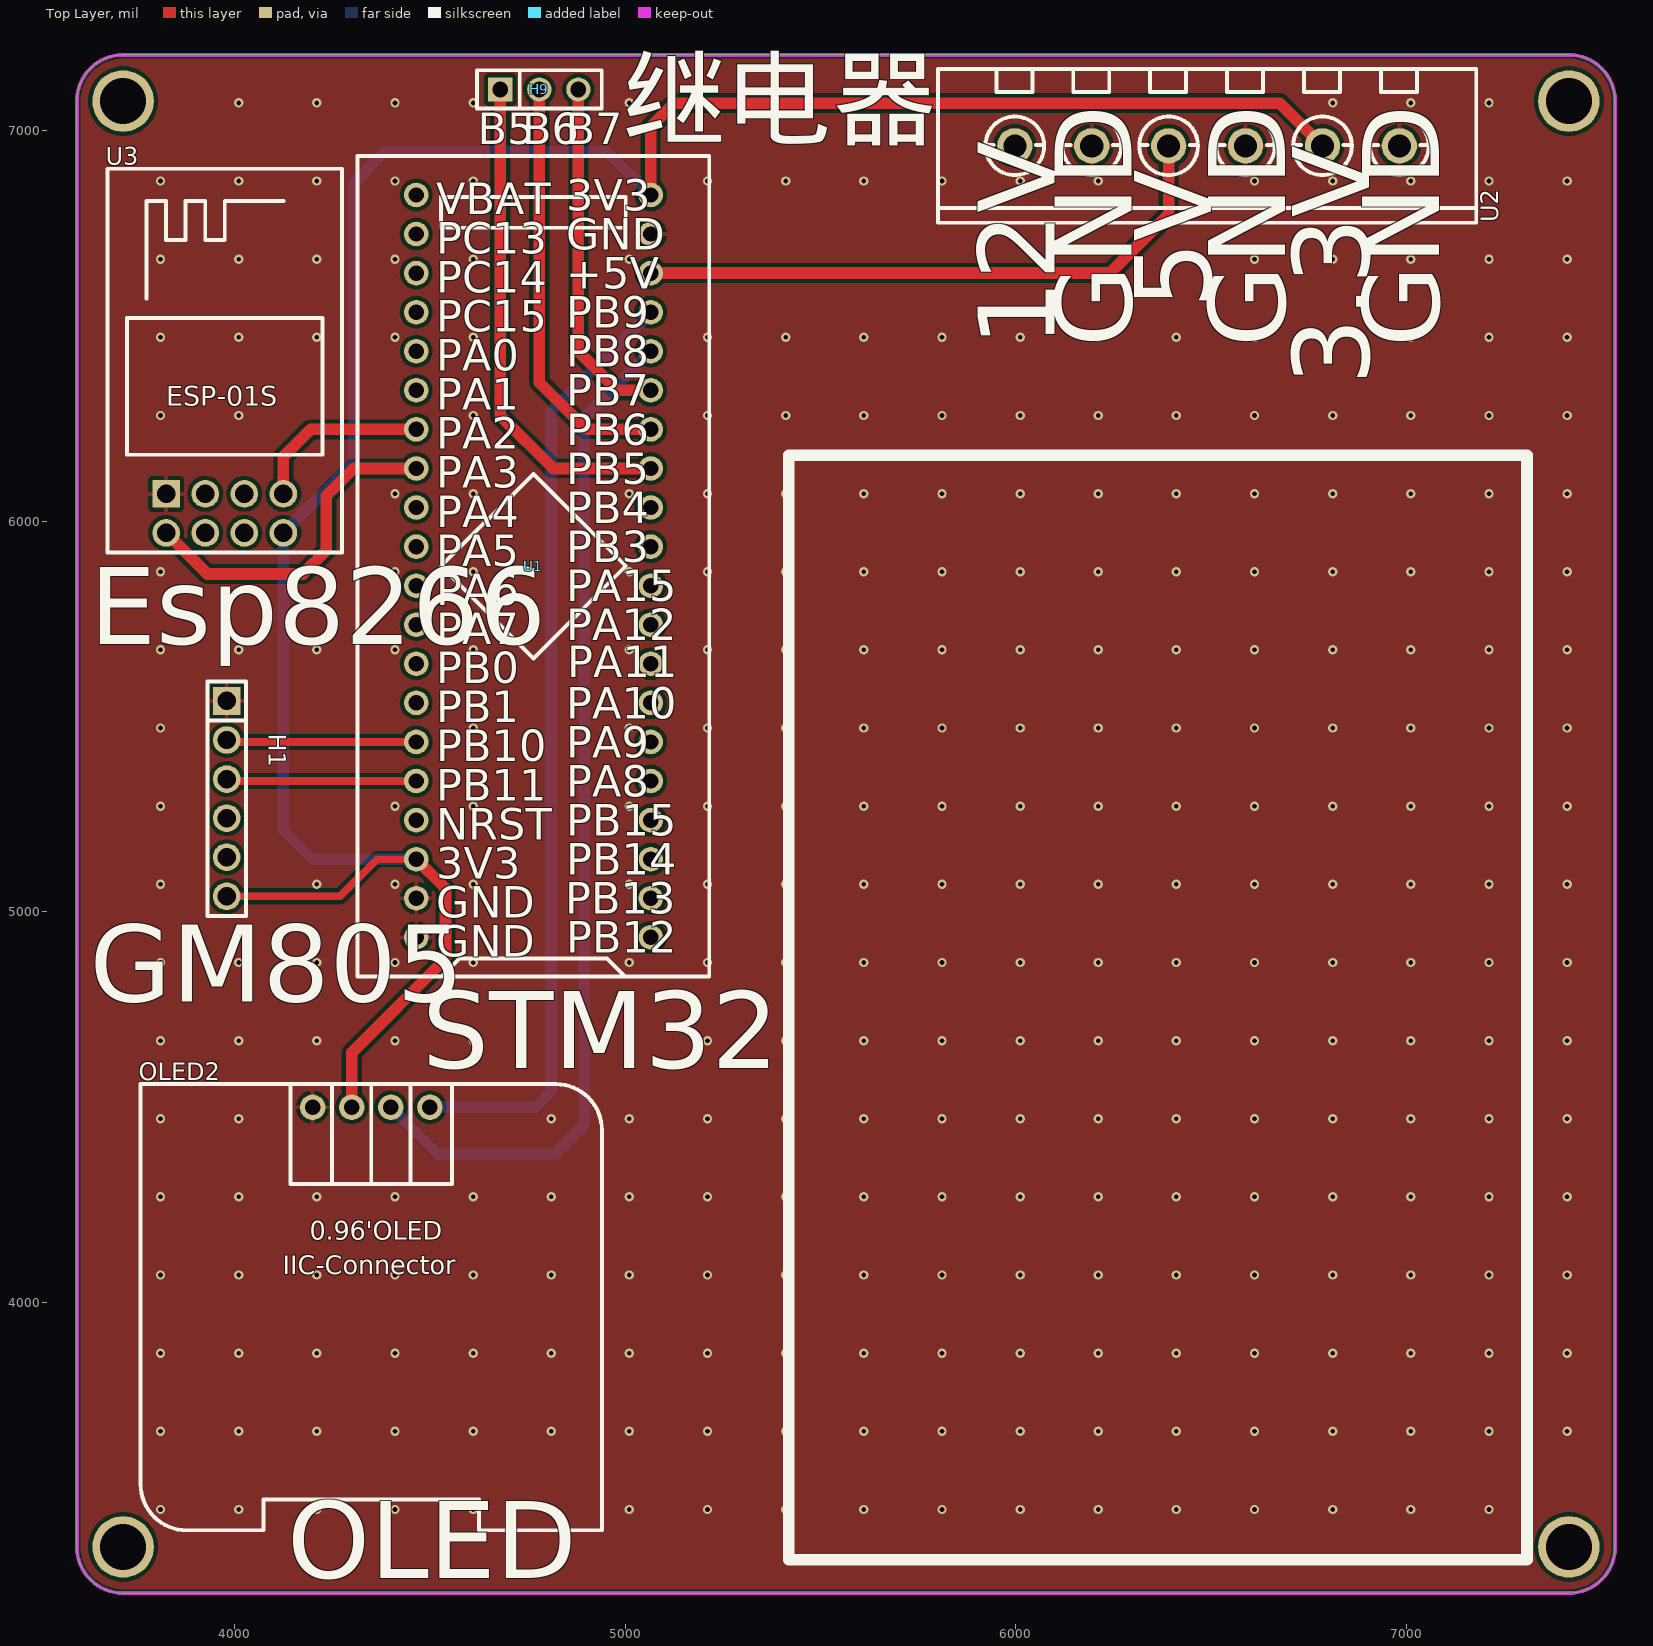
[diagram p0: Top Layer view]
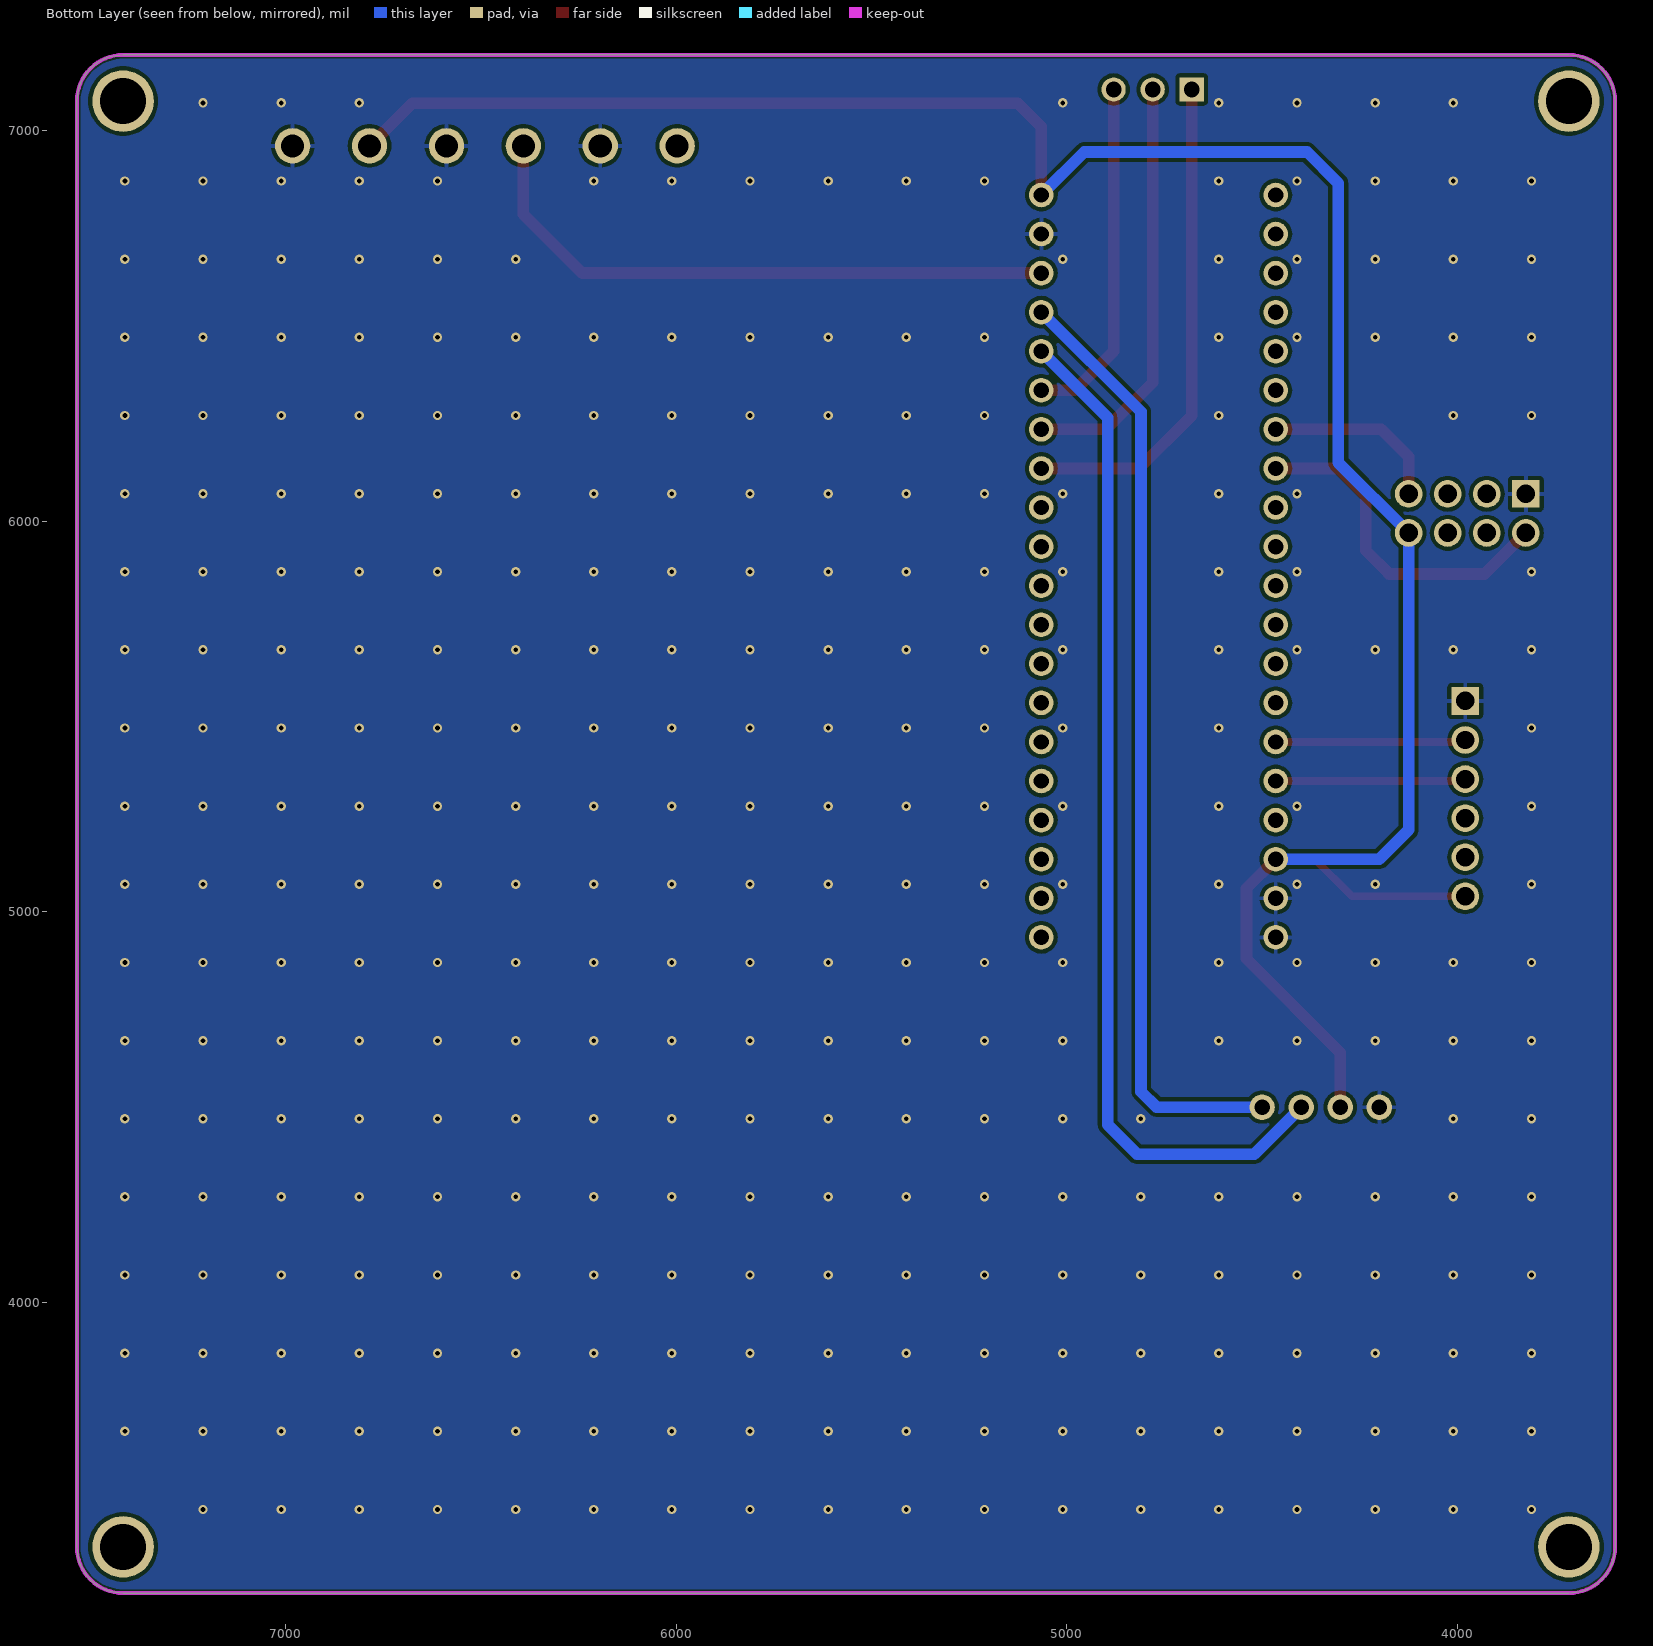
[diagram p1: Bottom Layer view, seen from below]
# Altium PCB MISC52106.pcbdoc
Units mil, origin at the board's own origin, x right, y up, seen from the top; angles counter-clockwise.
Board outline 3937.01 x 3937.01 mil, 2 copper layers (Top Layer, Bottom Layer), stack 62.206 mil thick; 6 components, 38 nets, 71 pads, 311 vias.

## Layer stack, top to bottom
Top Solder Mask Layer: solder mask 0.394, Dk 3.3
Top Layer: signal copper 1.379
Dielectric1: surface 59.449, FR4, Dk 4.5
Bottom Layer: signal copper 1.378
Bottom Solder Mask Layer: solder mask 0.394, Dk 3.3

## Board outline
3714.61,7193.5 ccw(c3714.61,7075.39) 3596.5,7075.39 3596.5,3374.61 ccw(c3714.61,3374.61) 3714.61,3256.5 7415.39,3256.5 ccw(c7415.39,3374.61) 7533.5,3374.61 7533.5,7075.39 ccw(c7415.39,7075.39) 7415.39,7193.5 3714.61,7193.5

## Design rules (kind name [scope] priority, off if disabled: settings)
BoardOutlineClearance copperThickness2oz_1 [All] p2 off: genericclearance=7.99 ignorepadtopadclearanceinfootprint=FALSE except(0: Arc-SplitContinuation Track-SplitContinuation SMDPad-SplitContinuation THPad-SplitContinuation Via-SplitContinuation Fill-SplitContinuation Region-SplitContinuation Poly-SplitContinuation Text-SplitContinuation Hole-SplitContinuation; 5.98: Arc-CutoutEdge Track-CutoutEdge SMDPad-CutoutEdge THPad-CutoutEdge Via-CutoutEdge Text-CutoutEdge; 6.9: Hole-OutlineEdge Hole-CutoutEdge; 10: Poly-OutlineEdge Poly-CutoutEdge; 11.81: Arc-OutlineEdge Track-OutlineEdge SMDPad-OutlineEdge THPad-OutlineEdge Via-OutlineEdge Fill-OutlineEdge Region-OutlineEdge Text-OutlineEdge Fill-CutoutEdge Region-CutoutEdge)
BoardOutlineClearance Plane_innerPlane_1 [All] p4 off: genericclearance=4.02 ignorepadtopadclearanceinfootprint=FALSE except(0: Arc-SplitContinuation Track-SplitContinuation SMDPad-SplitContinuation THPad-SplitContinuation Via-SplitContinuation Fill-SplitContinuation Region-SplitContinuation Poly-SplitContinuation Text-SplitContinuation Hole-SplitContinuation; 5.98: Arc-CutoutEdge Track-CutoutEdge SMDPad-CutoutEdge THPad-CutoutEdge Via-CutoutEdge Text-CutoutEdge; 6.9: Hole-OutlineEdge Hole-CutoutEdge; 10: Poly-OutlineEdge Poly-CutoutEdge; 11.81: Arc-OutlineEdge Track-OutlineEdge SMDPad-OutlineEdge THPad-OutlineEdge Via-OutlineEdge Fill-OutlineEdge Region-OutlineEdge Text-OutlineEdge Fill-CutoutEdge Region-CutoutEdge)
BoardOutlineClearance Copper_copperRegion_1 [All] p6 off: genericclearance=4.02 ignorepadtopadclearanceinfootprint=FALSE except(0: Arc-SplitContinuation Track-SplitContinuation SMDPad-SplitContinuation THPad-SplitContinuation Via-SplitContinuation Fill-SplitContinuation Region-SplitContinuation Poly-SplitContinuation Text-SplitContinuation Hole-SplitContinuation; 5.98: Arc-CutoutEdge Track-CutoutEdge SMDPad-CutoutEdge THPad-CutoutEdge Via-CutoutEdge Text-CutoutEdge; 6.9: Hole-OutlineEdge Hole-CutoutEdge; 10: Poly-OutlineEdge Poly-CutoutEdge; 11.81: Arc-OutlineEdge Track-OutlineEdge SMDPad-OutlineEdge THPad-OutlineEdge Via-OutlineEdge Fill-OutlineEdge Region-OutlineEdge Text-OutlineEdge Fill-CutoutEdge Region-CutoutEdge)
BoardOutlineClearance Copper_copperRegion_copperThickness1oz_1 [All] p8 off: genericclearance=4.02 ignorepadtopadclearanceinfootprint=FALSE except(0: Arc-SplitContinuation Track-SplitContinuation SMDPad-SplitContinuation THPad-SplitContinuation Via-SplitContinuation Fill-SplitContinuation Region-SplitContinuation Poly-SplitContinuation Text-SplitContinuation Hole-SplitContinuation; 5.98: Arc-CutoutEdge Track-CutoutEdge SMDPad-CutoutEdge THPad-CutoutEdge Via-CutoutEdge Text-CutoutEdge; 6.9: Hole-OutlineEdge Hole-CutoutEdge; 10: Poly-OutlineEdge Poly-CutoutEdge; 11.81: Arc-OutlineEdge Track-OutlineEdge SMDPad-OutlineEdge THPad-OutlineEdge Via-OutlineEdge Fill-OutlineEdge Region-OutlineEdge Text-OutlineEdge Fill-CutoutEdge Region-CutoutEdge)
BoardOutlineClearance Copper_copperRegion_Copper_copperRegion_1 [All] p10 off: genericclearance=4.02 ignorepadtopadclearanceinfootprint=FALSE except(0: Arc-SplitContinuation Track-SplitContinuation SMDPad-SplitContinuation THPad-SplitContinuation Via-SplitContinuation Fill-SplitContinuation Region-SplitContinuation Poly-SplitContinuation Text-SplitContinuation Hole-SplitContinuation; 5.98: Arc-CutoutEdge Track-CutoutEdge SMDPad-CutoutEdge THPad-CutoutEdge Via-CutoutEdge Text-CutoutEdge; 6.9: Hole-OutlineEdge Hole-CutoutEdge; 10: Poly-OutlineEdge Poly-CutoutEdge; 11.81: Arc-OutlineEdge Track-OutlineEdge SMDPad-OutlineEdge THPad-OutlineEdge Via-OutlineEdge Fill-OutlineEdge Region-OutlineEdge Text-OutlineEdge Fill-CutoutEdge Region-CutoutEdge)
BoardOutlineClearance copperThickness1oz_1 [All] p12: genericclearance=4.02 ignorepadtopadclearanceinfootprint=FALSE except(0: Arc-SplitContinuation Track-SplitContinuation SMDPad-SplitContinuation THPad-SplitContinuation Via-SplitContinuation Fill-SplitContinuation Region-SplitContinuation Poly-SplitContinuation Text-SplitContinuation Hole-SplitContinuation; 5.98: Arc-CutoutEdge Track-CutoutEdge SMDPad-CutoutEdge THPad-CutoutEdge Via-CutoutEdge Text-CutoutEdge; 6.9: Hole-OutlineEdge Hole-CutoutEdge; 10: Poly-OutlineEdge Poly-CutoutEdge; 11.81: Arc-OutlineEdge Track-OutlineEdge SMDPad-OutlineEdge THPad-OutlineEdge Via-OutlineEdge Fill-OutlineEdge Region-OutlineEdge Text-OutlineEdge Fill-CutoutEdge Region-CutoutEdge)
Clearance copperThickness2oz [All] p1 off: gap=7.99 ignorepadtopadclearanceinfootprint=FALSE except(5.98: SMDPad-Track SMDPad-SMDPad THPad-Track SMDPad-THPad THPad-THPad Track-Via SMDPad-Via THPad-Via Via-Via Fill-SMDPad Region-SMDPad Fill-THPad Region-THPad Fill-Via Region-Via Fill-Fill Fill-Region Region-Region Arc-Track Arc-SMDPad Arc-THPad Arc-Via Fill-Arc Region-Arc Arc-Arc Text-Track SMDPad-Text Text-THPad Text-Via Fill-Text Region-Text Arc-Text Text-Text; 6.9: Hole-Track Hole-SMDPad Hole-THPad Hole-Via Fill-Hole Region-Hole Hole-Arc Hole-Text; 10: Poly-Track Poly-SMDPad Poly-THPad Poly-Via Poly-Fill Poly-Region Poly-Poly Poly-Arc Poly-Text Poly-Hole; 11.81: Fill-Track Region-Track)
Clearance Plane_innerPlane [All] p3 off: gap=4.02 ignorepadtopadclearanceinfootprint=FALSE except(5.98: SMDPad-Track SMDPad-SMDPad THPad-Track SMDPad-THPad THPad-THPad Track-Via SMDPad-Via THPad-Via Via-Via Fill-SMDPad Region-SMDPad Fill-THPad Region-THPad Fill-Via Region-Via Fill-Fill Fill-Region Region-Region Arc-Track Arc-SMDPad Arc-THPad Arc-Via Fill-Arc Region-Arc Arc-Arc Text-Track SMDPad-Text Text-THPad Text-Via Fill-Text Region-Text Arc-Text Text-Text; 6.9: Hole-Track Hole-SMDPad Hole-THPad Hole-Via Fill-Hole Region-Hole Hole-Arc Hole-Text; 10: Poly-Track Poly-SMDPad Poly-THPad Poly-Via Poly-Fill Poly-Region Poly-Poly Poly-Arc Poly-Text Poly-Hole; 11.81: Fill-Track Region-Track)
Clearance Copper_copperRegion [All] p5 off: gap=4.02 ignorepadtopadclearanceinfootprint=FALSE except(5.98: SMDPad-Track SMDPad-SMDPad THPad-Track SMDPad-THPad THPad-THPad Track-Via SMDPad-Via THPad-Via Via-Via Fill-SMDPad Region-SMDPad Fill-THPad Region-THPad Fill-Via Region-Via Fill-Fill Fill-Region Region-Region Arc-Track Arc-SMDPad Arc-THPad Arc-Via Fill-Arc Region-Arc Arc-Arc Text-Track SMDPad-Text Text-THPad Text-Via Fill-Text Region-Text Arc-Text Text-Text; 6.9: Hole-Track Hole-SMDPad Hole-THPad Hole-Via Fill-Hole Region-Hole Hole-Arc Hole-Text; 10: Poly-Track Poly-SMDPad Poly-THPad Poly-Via Poly-Fill Poly-Region Poly-Poly Poly-Arc Poly-Text Poly-Hole; 11.81: Fill-Track Region-Track)
Clearance Copper_copperRegion_copperThickness1oz [All] p7 off: gap=4.02 ignorepadtopadclearanceinfootprint=FALSE except(5.98: SMDPad-Track SMDPad-SMDPad THPad-Track SMDPad-THPad THPad-THPad Track-Via SMDPad-Via THPad-Via Via-Via Fill-SMDPad Region-SMDPad Fill-THPad Region-THPad Fill-Via Region-Via Fill-Fill Fill-Region Region-Region Arc-Track Arc-SMDPad Arc-THPad Arc-Via Fill-Arc Region-Arc Arc-Arc Text-Track SMDPad-Text Text-THPad Text-Via Fill-Text Region-Text Arc-Text Text-Text; 6.9: Hole-Track Hole-SMDPad Hole-THPad Hole-Via Fill-Hole Region-Hole Hole-Arc Hole-Text; 10: Poly-Track Poly-SMDPad Poly-THPad Poly-Via Poly-Fill Poly-Region Poly-Poly Poly-Arc Poly-Text Poly-Hole; 11.81: Fill-Track Region-Track)
Clearance Copper_copperRegion_Copper_copperRegion [All] p9 off: gap=4.02 ignorepadtopadclearanceinfootprint=FALSE except(5.98: SMDPad-Track SMDPad-SMDPad THPad-Track SMDPad-THPad THPad-THPad Track-Via SMDPad-Via THPad-Via Via-Via Fill-SMDPad Region-SMDPad Fill-THPad Region-THPad Fill-Via Region-Via Fill-Fill Fill-Region Region-Region Arc-Track Arc-SMDPad Arc-THPad Arc-Via Fill-Arc Region-Arc Arc-Arc Text-Track SMDPad-Text Text-THPad Text-Via Fill-Text Region-Text Arc-Text Text-Text; 6.9: Hole-Track Hole-SMDPad Hole-THPad Hole-Via Fill-Hole Region-Hole Hole-Arc Hole-Text; 10: Poly-Track Poly-SMDPad Poly-THPad Poly-Via Poly-Fill Poly-Region Poly-Poly Poly-Arc Poly-Text Poly-Hole; 11.81: Fill-Track Region-Track)
Clearance copperThickness1oz [All] p11: gap=4.02 ignorepadtopadclearanceinfootprint=FALSE except(5.98: SMDPad-Track SMDPad-SMDPad THPad-Track SMDPad-THPad THPad-THPad Track-Via SMDPad-Via THPad-Via Via-Via Fill-SMDPad Region-SMDPad Fill-THPad Region-THPad Fill-Via Region-Via Fill-Fill Fill-Region Region-Region Arc-Track Arc-SMDPad Arc-THPad Arc-Via Fill-Arc Region-Arc Arc-Arc Text-Track SMDPad-Text Text-THPad Text-Via Fill-Text Region-Text Arc-Text Text-Text; 6.9: Hole-Track Hole-SMDPad Hole-THPad Hole-Via Fill-Hole Region-Hole Hole-Arc Hole-Text; 10: Poly-Track Poly-SMDPad Poly-THPad Poly-Via Poly-Fill Poly-Region Poly-Poly Poly-Arc Poly-Text Poly-Hole; 11.81: Fill-Track Region-Track)
DiffPairsRouting differentialPair [All] p1: maxlimit=6 minlimit=6 mostfreqgap=6 toplayer_minwidth=5 toplayer_prefwidth=10 toplayer_maxwidth=100 toplayer_mingap=6 toplayer_prefgap=6 toplayer_maxgap=6 bottomlayer_minwidth=5 bottomlayer_prefwidth=10 bottomlayer_maxwidth=100 bottomlayer_mingap=6 bottomlayer_prefgap=6 bottomlayer_maxgap=6 maxuncoupledlength=10
HoleToHoleClearance otherClearance [All] p1: gap=11.81 allowstackedmicrovias=TRUE
Length netLength [All] p1: minlimit=0 maxlimit=0
PasteMaskExpansion pasteMaskExpansion [All] p1: expansion=0
PlaneConnect innerPlane [All] p1: planeconnectstyle=Relief reliefexpansion=20 reliefentries=4 reliefconductorwidth=10 reliefairgap=10
PolygonConnect copperRegion_copperThickness1oz [All] p1 off: connectstyle=Relief reliefconductorwidth=10 reliefentries=4 polygonreliefangle="90 Angle" airgapwidth=10 via.connectstyle=Relief via.reliefconductorwidth=10 via.reliefentries=4 via.polygonreliefangle="90 Angle" via.airgapwidth=10
PolygonConnect copperRegion_Copper_copperRegion [All] p2 off: connectstyle=Relief reliefconductorwidth=10 reliefentries=4 polygonreliefangle="90 Angle" airgapwidth=10 via.connectstyle=Relief via.reliefconductorwidth=10 via.reliefentries=4 via.polygonreliefangle="90 Angle" via.airgapwidth=10
PolygonConnect copperRegion [All] p3: connectstyle=Relief reliefconductorwidth=10 reliefentries=4 polygonreliefangle="90 Angle" airgapwidth=10 via.connectstyle=Relief via.reliefconductorwidth=10 via.reliefentries=4 via.polygonreliefangle="90 Angle" via.airgapwidth=10
RoutingVias viaSize [All] p1: holewidth=12.01 width=24.02 viastyle="Through Hole" minholewidth=11.81 minwidth=19.68 maxholewidth=248.03 maxwidth=393.7
SolderMaskExpansion solderMaskExpansion [IsVia] p1: expansion=-1000 istentingtop=TRUE
SolderMaskExpansion solderMaskExpansion [All] p2: expansion=2 istentingtop=FALSE
Width copperThickness2oz_2 [All] p1 off: maxlimit=100 minlimit=8 preferedwidth=10
Width copperThickness1oz_2 [All] p2: maxlimit=100 minlimit=5 preferedwidth=10

## Components (designator, comment, footprint, x,y, rotation, side; value= is the part's Value field where it differs from the comment)
H1 "" HDR-TH_6P-P2.54-V-M-1 3980,5290 r270 top
H9 "" HDR-TH_3P-P2.54-V-F 4780,7105 r0 top
OLED2 "" 0.96OLED_4P 4350,4500 r0 top
U1 "STM32F103C8T6-Card" CONN-TH_L53.3-W22.9_STM32F103C8T6-CARD 4765,5885 r90 top
U2 "LG128V 5.08 6P180度螺丝用十字带一字型" CONN-TH_6P-P5.00_LG128V 6489.22,6960.78 r180 top
U3 "ESP-01S" WIFIM-TH_ESP-01S 3975,6020 r0 top

## Footprints (in the part's own frame and the unit in brackets; to place one, negate y for a bottom-side part, rotate by r counter-clockwise, add the part's x,y. Pads: shape width x height; smd on the part's side, far side on the other; paste and mask are expansions set on the pad)
0.96OLED_4P [mm]
  round 1.65 hole 1 copper offset 0,0: 1(-3.81,-0.001) 2(-1.27,0.002) 3(1.27,0.002) 4(3.81,0.002)
  silkscreen extent -15,-27.5 15,1.5
CONN-TH_6P-P5.00_LG128V [mm]
  round 2.3 hole 1.5 paste+0 mask+0.05: 1(-12.5,0) 2(-7.5,0) 3(-2.5,0) 4(2.5,0) 5(7.5,0) 6(12.5,0)
  silkscreen extent -17.5,-5 17.5,5
CONN-TH_L53.3-W22.9_STM32F103C8T6-CARD [mm]
  round 1.6 hole 1: 1(-24.13,-7.62) 2(-21.59,-7.62) 3(-19.05,-7.62) 4(-16.51,-7.62) 5(-13.97,-7.62) 6(-11.43,-7.62) 7(-8.89,-7.62) 8(-6.35,-7.62) 9(-3.81,-7.62) 10(-1.27,-7.62) 11(1.27,-7.62) 12(3.81,-7.62) 13(6.35,-7.62) 14(8.89,-7.62) 15(11.43,-7.62) 16(13.97,-7.62) 17(16.51,-7.62) 18(19.05,-7.62) 19(21.59,-7.62) 20(24.13,-7.62) 21(24.13,7.62) 22(21.59,7.62) 23(19.05,7.62) 24(16.51,7.62) 25(13.97,7.62) 26(11.43,7.62) 27(8.89,7.62) 28(6.35,7.62) 29(3.81,7.62) 30(1.27,7.62) 31(-1.27,7.62) 32(-3.81,7.62) 33(-6.35,7.62) 34(-8.89,7.62) 35(-11.43,7.62) 36(-13.97,7.62) 37(-16.51,7.62) 38(-19.05,7.62) 39(-21.59,7.62) 40(-24.13,7.62)
  silkscreen extent -26.67,-11.43 26.67,11.43
HDR-TH_3P-P2.54-V-F [mil]
  rect 62x62 hole 40.16: 1(-100,0)
  round 62 hole 40.16: 2(0,0) 3(100,0)
  silkscreen extent -160,-49 160,49
HDR-TH_6P-P2.54-V-M-1 [mm]
  rect 1.8x1.8 hole 1.2: 1(-6.35,0)
  round 1.8 hole 1.2: 2(-3.81,0) 3(-1.27,0) 4(1.27,0) 5(3.81,0) 6(6.35,0)
  silkscreen extent -7.62,-1.25 7.62,1.25
WIFIM-TH_ESP-01S [mm]
  rect 1.8x1.8 hole 1.2: 1(-3.81,1.27)
  round 1.8 hole 1.2: 2(-1.27,1.27) 3(1.27,1.27) 4(3.81,1.27) 5(3.81,-1.27) 6(1.27,-1.27) 7(-1.27,-1.27) 8(-3.81,-1.27)
  silkscreen extent -7.62,-2.54 7.62,22.4

## Free pads (board coordinates)
  round 157.48 hole 118.11: 1(3714.61,7075.39) 1(3714.61,3374.61) 1(7415.39,7075.39) 1(7415.39,3374.61)

## Via types
v1: diameter 24.02, hole 12, Top Layer to Bottom Layer, 311 vias

## Nets (pads, with @x,y where several pads share a name; then routed paths per layer and width w, separated by ;. In a path a pad name is that pad's centre, name@x,y a point inside that pad or via, vN(x,y) a via of type N, cw(c..) or ccw(c..) an arc to the next point about the centre after c; other vN are vias at no path point)
12V: U2.6
+5V: U1.18 U2.4 | length 1563.2
  Top Layer w30: U1.18 6240,6635 6390.79,6785.79 U2.4
GND: H1.1 OLED2.1 U1.19 U1.39 U1.40 U2.1 U2.3 U2.5 U3.1
  other v1: 3810.6,3470.6 4010.6,3470.6 4210.6,3470.6 4410.6,3470.6 4610.6,3470.6 4810.6,3470.6 5010.6,3470.6 5210.6,3470.6 5410.6,3470.6 5610.6,3470.6 5810.6,3470.6 6010.6,3470.6 6210.6,3470.6 6410.6,3470.6 6610.6,3470.6 6810.6,3470.6 7010.6,3470.6 7210.6,3470.6 3810.6,3670.6 4010.6,3670.6 4210.6,3670.6 4410.6,3670.6 4610.6,3670.6 4810.6,3670.6 5010.6,3670.6 5210.6,3670.6 5410.6,3670.6 5610.6,3670.6 5810.6,3670.6 6010.6,3670.6 6210.6,3670.6 6410.6,3670.6 6610.6,3670.6 6810.6,3670.6 7010.6,3670.6 7210.6,3670.6 7410.6,3670.6 3810.6,3870.6 4010.6,3870.6 4210.6,3870.6 4410.6,3870.6 4610.6,3870.6 4810.6,3870.6 5010.6,3870.6 5210.6,3870.6 5410.6,3870.6 5610.6,3870.6 5810.6,3870.6 6010.6,3870.6 6210.6,3870.6 6410.6,3870.6 6610.6,3870.6 6810.6,3870.6 7010.6,3870.6 7210.6,3870.6 7410.6,3870.6 3810.6,4070.6 4010.6,4070.6 4210.6,4070.6 4410.6,4070.6 4610.6,4070.6 4810.6,4070.6 5010.6,4070.6 5210.6,4070.6 5410.6,4070.6 5610.6,4070.6 5810.6,4070.6 6010.6,4070.6 6210.6,4070.6 6410.6,4070.6 6610.6,4070.6 6810.6,4070.6 7010.6,4070.6 7210.6,4070.6 7410.6,4070.6 3810.6,4270.6 4010.6,4270.6 4210.6,4270.6 4410.6,4270.6 4610.6,4270.6 4810.6,4270.6 5010.6,4270.6 5210.6,4270.6 5410.6,4270.6 5610.6,4270.6 5810.6,4270.6 6010.6,4270.6 6210.6,4270.6 6410.6,4270.6 6610.6,4270.6 6810.6,4270.6 7010.6,4270.6 7210.6,4270.6 7410.6,4270.6 3810.6,4470.6 4010.6,4470.6 4810.6,4470.6 5010.6,4470.6 5210.6,4470.6 5410.6,4470.6 5610.6,4470.6 5810.6,4470.6 6010.6,4470.6 6210.6,4470.6 6410.6,4470.6 6610.6,4470.6 6810.6,4470.6 7010.6,4470.6 7210.6,4470.6 7410.6,4470.6 3810.6,4670.6 4010.6,4670.6 4210.6,4670.6 4410.6,4670.6 4610.6,4670.6 5010.6,4670.6 5210.6,4670.6 5410.6,4670.6 5610.6,4670.6 5810.6,4670.6 6010.6,4670.6 6210.6,4670.6 6410.6,4670.6 6610.6,4670.6 6810.6,4670.6 7010.6,4670.6 7210.6,4670.6 7410.6,4670.6 3810.6,4870.6 4010.6,4870.6 4210.6,4870.6 4410.6,4870.6 4610.6,4870.6 5010.6,4870.6 5210.6,4870.6 5410.6,4870.6 5610.6,4870.6 5810.6,4870.6 6010.6,4870.6 6210.6,4870.6 6410.6,4870.6 6610.6,4870.6 6810.6,4870.6 7010.6,4870.6 7210.6,4870.6 7410.6,4870.6 3810.6,5070.6 4210.6,5070.6 4410.6,5070.6 4610.6,5070.6 5010.6,5070.6 5210.6,5070.6 5410.6,5070.6 5610.6,5070.6 5810.6,5070.6 6010.6,5070.6 6210.6,5070.6 6410.6,5070.6 6610.6,5070.6 6810.6,5070.6 7010.6,5070.6 7210.6,5070.6 7410.6,5070.6 3810.6,5270.6 4410.6,5270.6 4610.6,5270.6 5010.6,5270.6 5210.6,5270.6 5410.6,5270.6 5610.6,5270.6 5810.6,5270.6 6010.6,5270.6 6210.6,5270.6 6410.6,5270.6 6610.6,5270.6 6810.6,5270.6 7010.6,5270.6 7210.6,5270.6 7410.6,5270.6 3810.6,5470.6 4610.6,5470.6 5010.6,5470.6 5210.6,5470.6 5410.6,5470.6 5610.6,5470.6 5810.6,5470.6 6010.6,5470.6 6210.6,5470.6 6410.6,5470.6 6610.6,5470.6 6810.6,5470.6 7010.6,5470.6 7210.6,5470.6 7410.6,5470.6 3810.6,5670.6 4010.6,5670.6 4210.6,5670.6 4410.6,5670.6 4610.6,5670.6 5010.6,5670.6 5210.6,5670.6 5410.6,5670.6 5610.6,5670.6 5810.6,5670.6 6010.6,5670.6 6210.6,5670.6 6410.6,5670.6 6610.6,5670.6 6810.6,5670.6 7010.6,5670.6 7210.6,5670.6 7410.6,5670.6 3810.6,5870.6 4410.6,5870.6 4610.6,5870.6 5010.6,5870.6 5210.6,5870.6 5410.6,5870.6 5610.6,5870.6 5810.6,5870.6 6010.6,5870.6 6210.6,5870.6 6410.6,5870.6 6610.6,5870.6 6810.6,5870.6 7010.6,5870.6 7210.6,5870.6 7410.6,5870.6 4410.6,6070.6 4610.6,6070.6 5010.6,6070.6 5210.6,6070.6 5410.6,6070.6 5610.6,6070.6 5810.6,6070.6 6010.6,6070.6 6210.6,6070.6 6410.6,6070.6 6610.6,6070.6 6810.6,6070.6 7010.6,6070.6 7210.6,6070.6 7410.6,6070.6 3810.6,6270.6 4010.6,6270.6 4610.6,6270.6 5210.6,6270.6 5410.6,6270.6 5610.6,6270.6 5810.6,6270.6 6010.6,6270.6 6210.6,6270.6 6410.6,6270.6 6610.6,6270.6 6810.6,6270.6 7010.6,6270.6 7210.6,6270.6 7410.6,6270.6 3810.6,6470.6 4010.6,6470.6 4210.6,6470.6 4410.6,6470.6 4610.6,6470.6 5210.6,6470.6 5410.6,6470.6 5610.6,6470.6 5810.6,6470.6 6010.6,6470.6 6210.6,6470.6 6410.6,6470.6 6610.6,6470.6 6810.6,6470.6 7010.6,6470.6 7210.6,6470.6 7410.6,6470.6 3810.6,6670.6 4010.6,6670.6 4210.6,6670.6 4410.6,6670.6 4610.6,6670.6 5010.6,6670.6 6410.6,6670.6 6610.6,6670.6 6810.6,6670.6 7010.6,6670.6 7210.6,6670.6 7410.6,6670.6 3810.6,6870.6 4010.6,6870.6 4210.6,6870.6 4410.6,6870.6 4610.6,6870.6 5210.6,6870.6 5410.6,6870.6 5610.6,6870.6 5810.6,6870.6 6010.6,6870.6 6210.6,6870.6 6610.6,6870.6 6810.6,6870.6 7010.6,6870.6 7210.6,6870.6 7410.6,6870.6 4010.6,7070.6 4210.6,7070.6 4410.6,7070.6 4610.6,7070.6 5010.6,7070.6 6810.6,7070.6 7010.6,7070.6 7210.6,7070.6
NRST: U1.37
PA0: U1.25
PA1: U1.26
PA2: U1.27 U3.4 | length 464
  Top Layer w30: U3.4 4125,6165 4195,6235 U1.27
PA3: U1.28 U3.8 | length 877.3
  Top Layer w30: U3.8 3930,5865 4175,5865 4235,5925 4235,6065 4305,6135 U1.28
PA4: U1.29
PA5: U1.30
PA6: U1.31
PA7: U1.32
PA8: U1.5
PA9: U1.6
PA10: U1.7
PA11: U1.8
PA12: U1.9
PA15: U1.10
PB0: U1.33
PB1: U1.34
PB3: U1.11
PB4: U1.12
PB5: H9.1 U1.13 | length 1275.9
  Top Layer w30: H9.1 4680,6270 4815,6135 U1.13
PB6: H9.2 U1.14 | length 1084.7
  Top Layer w30: H9.2 4780,6355 4900,6235 U1.14
PB7: H9.3 U1.15 | length 896.4
  Top Layer w30: H9.3 4880,6435 4980,6335 U1.15
PB8: OLED2.3 U1.16 | length 2626.2
  Bottom Layer w30: OLED2.3@4400,4500.05 4520.05,4380 4820,4380 4895,4455 4895,6265 U1.16
PB9: OLED2.4 U1.17 | length 2427.2
  Bottom Layer w30: OLED2.4@4500,4500.05 4770.05,4500.05 4810,4540 4810,6280 U1.17
PB10: H1.2 U1.35 | length 487.1
  Top Layer w20: H1.2 3985,5435 U1.35
PB11: H1.3 U1.36 | length 487.1
  Top Layer w20: H1.3 3985,5335 U1.36
PB12: U1.1
PB13: U1.2
PB14: U1.3
PB15: U1.4
PC13: U1.22
PC14: U1.23
PC15: U1.24
VBAT: U1.21
VCC: H1.6 OLED2.2 U1.20 U1.38 U2.2 U3.5 | length 6193.7
  Top Layer w20: H1.6 4270,5040 4365,5135 U1.38
  Top Layer w30: OLED2.2@4300,4500.05 4300,4640 4540,4880 4540,5060 U1.38 ; U1.20 5065,7010 5125,7070 6675.28,7070 U2.2
  Bottom Layer w30: U1.38 4200,5135 4125,5210 U3.5 4305,6150 4305,6865 4385,6945 4955,6945 U1.20
pads on no net: H1.4 H1.5 U3.2 U3.3 U3.6 U3.7

## Polygon pours and split planes (outlines as drawn)
GND on Bottom Layer (solid, remove dead copper, pour order 2): 3525,7260 3525,3095 7700,3095 7700,7260
GND on Top Layer (solid, remove dead copper, pour order 2): 3000,7415 3000,3000 7930,3000 7930,7415

## Keep-outs
Board Outline Layer:
  the board outline again, w10

## Silkscreen, mask and mechanical layers (free items; w line width, h text height)
Top Silkscreen Layer:
  lines w30: 5418.5,3341.73 7308.27,3341.73 7308.27,6168.5 5418.5,6168.5 5418.5,3341.73
  text "继电器" at 4990,6985 h196.85
  text "B5" at 4622.7,6965 h80
  text "B6" at 4736.3,6965 h80
  text "B7" at 4847.7,6965 h80
  text "3V3" at 4849.16,6795 h80
  text "VBAT" at 4515.95,6785 h80
  text "GND" at 4849.16,6695 h80
  text "PC13" at 4515.95,6685 h80
  text "+5V" at 4849.16,6595 h80
  text "PC14" at 4515.95,6585 h80
  text "5V" at 6500.22,6544.21 h196.85 r90
  text "PB9" at 4849.16,6495 h80
  text "PC15" at 4515.95,6485 h80
  text "12V" at 6099.22,6445.78 h196.85 r90
  text "GND" at 6296.07,6445.78 h196.85 r90
  text "GND" at 6689.77,6445.78 h196.85 r90
  text "GND" at 7083.47,6445.78 h196.85 r90
  text "PB8" at 4849.16,6395 h80
  text "PA0" at 4515.95,6385 h80
  text "3.3V" at 6904.22,6347.36 h196.85 r90
  text "PB7" at 4849.16,6295 h80
  text "PA1" at 4515.95,6285 h80
  text "PB6" at 4849.16,6195 h80
  text "PA2" at 4515.95,6185 h80
  text "PB5" at 4849.16,6095 h80
  text "PA3" at 4515.95,6085 h80
  text "PB4" at 4849.16,5995 h80
  text "PA4" at 4515.95,5985 h80
  text "PB3" at 4849.16,5895 h80
  text "PA5" at 4515.95,5885 h80
  text "PA15" at 4849.16,5795 h80
  text "PA6" at 4515.95,5785 h80
  text "PA12" at 4849.16,5695 h80
  text "Esp8266" at 3630,5685 h196.85
  text "PA7" at 4515.95,5685 h80
  text "PA11" at 4850.95,5600 h80
  text "PB0" at 4515.95,5585 h80
  text "PA10" at 4849.16,5495 h80
  text "PB1" at 4515.95,5485 h80
  text "PA9" at 4849.16,5395 h80
  text "PB10" at 4515.95,5385 h80
  text "PA8" at 4849.16,5295 h80
  text "PB11" at 4515.95,5285 h80
  text "PB15" at 4849.16,5195 h80
  text "NRST" at 4515.95,5185 h80
  text "PB14" at 4849.16,5095 h80
  text "3V3" at 4515.95,5085 h80
  text "PB13" at 4845.95,4995 h80
  text "GND" at 4515.95,4985 h80
  text "PB12" at 4849.16,4895 h80
  text "GND" at 4515.95,4885 h80
  text "GM805" at 3630,4770 h196.85
  text "STM32" at 4480,4600 h196.85
  text "OLED" at 4135,3295 h196.85